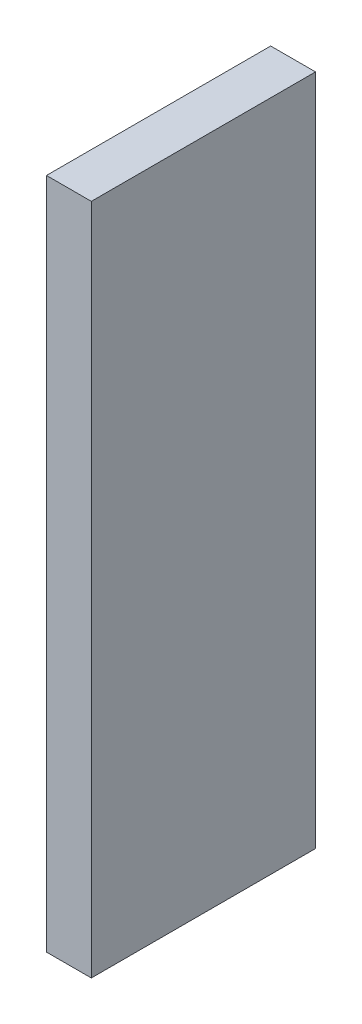
from build123d import *

# Parameters (mm, degrees)
SKETCH_1_W      = 20
SKETCH_1_H      = 60
EXTRUDE_1_DEPTH = 4


with BuildPart() as part:
    # 草图1 → 凸台-拉伸1 (new body)
    with BuildSketch(Plane(origin=(0, 0, 0), x_dir=(0, 0, -1), z_dir=(1, 0, 0))):
        with Locations((10, 30)):
            Rectangle(SKETCH_1_W, SKETCH_1_H)
    extrude(amount=EXTRUDE_1_DEPTH)


solid = part.part
